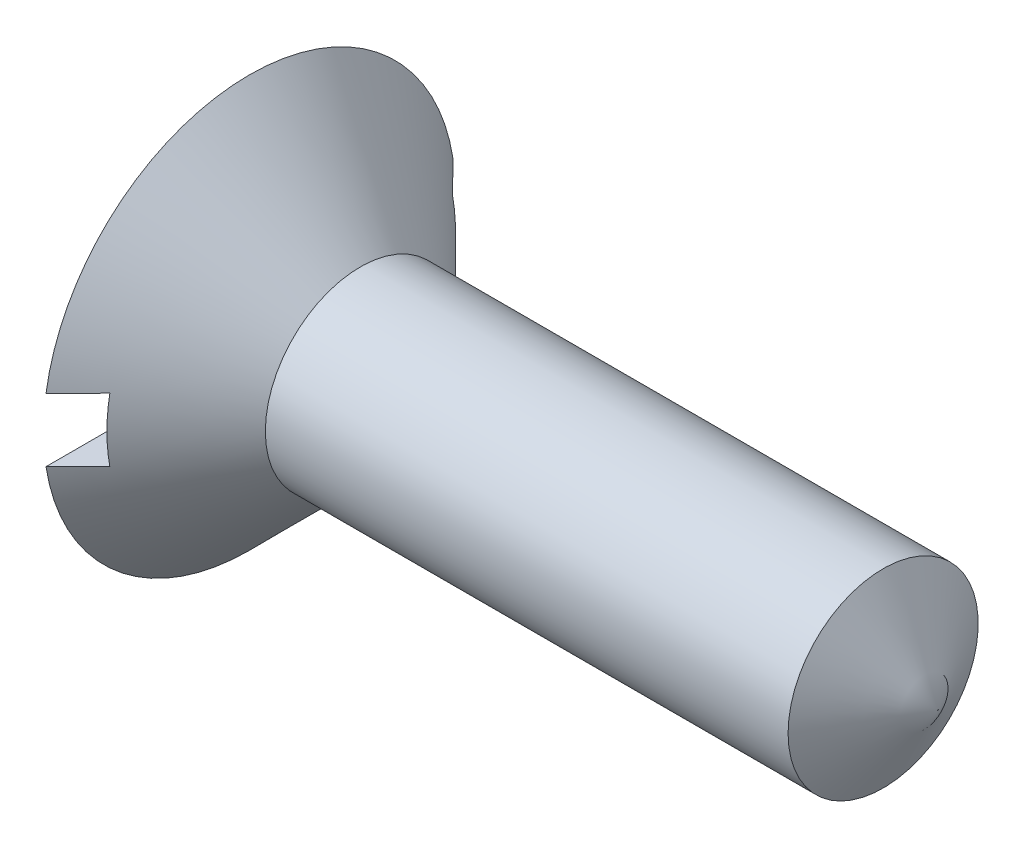
SolidWorks part; units mm, degrees
ref_plane "Front Plane" through (0, 0, 0) normal (0, 0, 1) x (1, 0, 0)
ref_plane "Top Plane" through (0, 0, 0) normal (0, 1, 0) x (1, 0, 0)
ref_plane "Right Plane" through (0, 0, 0) normal (1, 0, 0) x (0, 0, -1)
sketch "Sketch1" plane through (0, 0, 0) normal (0, 0, 1) x (1, 0, 0)
  line L0 (0, 0) -> (25.2699, 0) construction
  line L1 (0, 0) -> (0, 6.5)
  line L2 (0, 6.5) -> (3.5, 3)
  line L3 (3.5, 3) -> (20, 3)
  line L4 (20, 3) -> (21.7321, 0)
  line L5 (0, 0) -> (21.7321, 0)
  dimension "D1" = 45
  dimension "D2" = 20
  dimension "D3" = 3
  dimension "D4" = 60
  dimension "D5" = 6.5
revolve "Revolve1" add sketch "Sketch1" angle 360 about L0
sketch "Sketch2" plane through (0, 0, 0) normal (0, 0, 1) x (1, 0, 0)
  line L1 (-1, -1) -> (1, -1)
  line L2 (-1, -1) -> (-1, 1)
  line L3 (-1, 1) -> (1, 1)
  line L4 (1, -1) -> (1, 1)
  line L5 (-1, -1) -> (1, 1) construction
  line L6 (-1, 1) -> (1, -1) construction
  point P0 (0, 0)
  dimension "D1" = 2
  dimension "D2" = 1
extrude "Cut-Extrude1" cut sketch "Sketch2" along normal blind 12 and the other way blind 10
